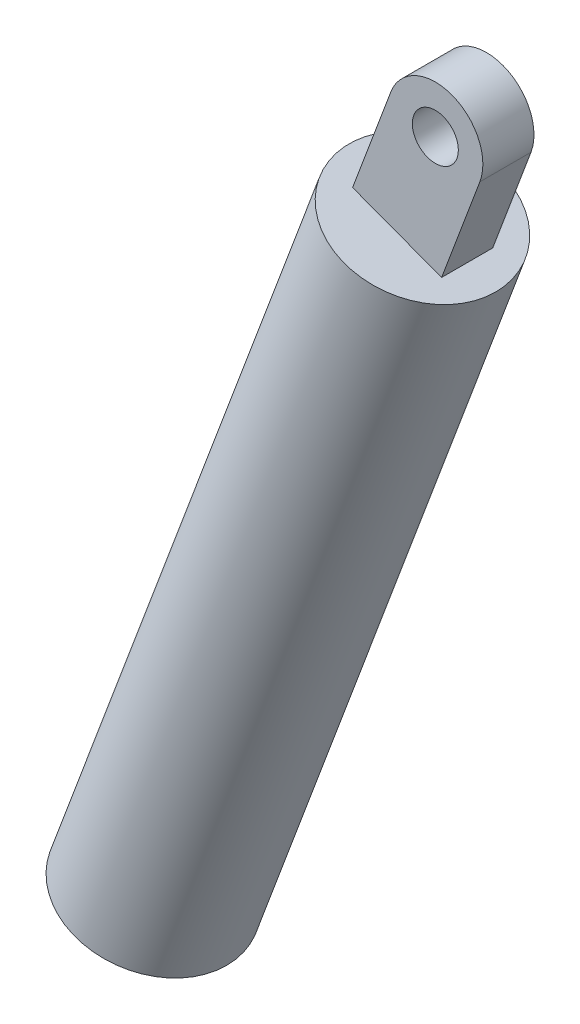
SolidWorks part; units mm, degrees
ref_plane "Front Plane" through (0, 0, 0) normal (0, 0, 1) x (1, 0, 0)
ref_plane "Top Plane" through (0, 0, 0) normal (0, 1, 0) x (1, 0, 0)
ref_plane "Right Plane" through (0, 0, 0) normal (1, 0, 0) x (0, 0, -1)
sketch "Sketch1" plane through (135.9071, 362.4686, 0) normal (-0.3511, -0.9363, 0) x (0.9363, -0.3511, 0)
  arc A2 (546.1928, 2365.7196) -> (546.1928, 2304.4208) centre (546.1928, 2335.0702) ccw
  arc A3 (546.1928, 2304.4208) -> (546.1928, 2365.7196) centre (546.1928, 2335.0702) ccw
  arc A4 (546.1928, 2365.7196) -> (546.1928, 2304.4208) centre (546.1928, 2335.0702) ccw
  arc A5 (546.1928, 2304.4208) -> (546.1928, 2365.7196) centre (546.1928, 2335.0702) ccw
  dimension "D1" = 0
extrude "Boss-Extrude1" add sketch "Sketch1" against normal up to vertex (300 mm away)
sketch "Sketch2" plane through (0, 0, 2344.9845) normal (0, 0, 1) x (1, 0, 0)
  line L3 (750.1999, 498.0383) -> (735.2415, 458.1437)
  line L4 (735.2415, 458.1437) -> (770.0712, 445.0844)
  line L5 (770.0712, 445.0844) -> (785.0296, 484.9789)
  line L6 (750.1999, 498.0383) -> (735.2415, 458.1437)
  line L7 (735.2415, 458.1437) -> (770.0712, 445.0844)
  line L8 (770.0712, 445.0844) -> (785.0296, 484.9789)
  arc A0 (760.636, 485.8256) -> (774.5936, 497.1915) centre (767.6148, 491.5086) ccw construction
  arc A1 (785.0296, 484.9789) -> (750.1999, 498.0383) centre (767.6148, 491.5086) ccw
  arc A2 (785.0296, 484.9789) -> (750.1999, 498.0383) centre (767.6148, 491.5086) ccw
  arc A3 (774.5936, 497.1915) -> (760.636, 485.8256) centre (767.6148, 491.5086) ccw construction
  arc A4 (760.636, 485.8256) -> (774.5936, 497.1915) centre (767.6148, 491.5086) ccw
  arc A5 (774.5936, 497.1915) -> (760.636, 485.8256) centre (767.6148, 491.5086) ccw
  dimension "D1" = 0
extrude "Boss-Extrude2" add sketch "Sketch2" against normal up to vertex (20 mm away)
sketch "Sketch3" plane through (135.9071, 362.4686, 0) normal (-0.3511, -0.9363, 0) x (0.9363, -0.3511, 0)
  circle A0 centre (546.1928, 2333.8341) radius 20
  dimension "D1" = 40
extrude "Cut-Extrude1" cut sketch "Sketch3" against normal blind 260
